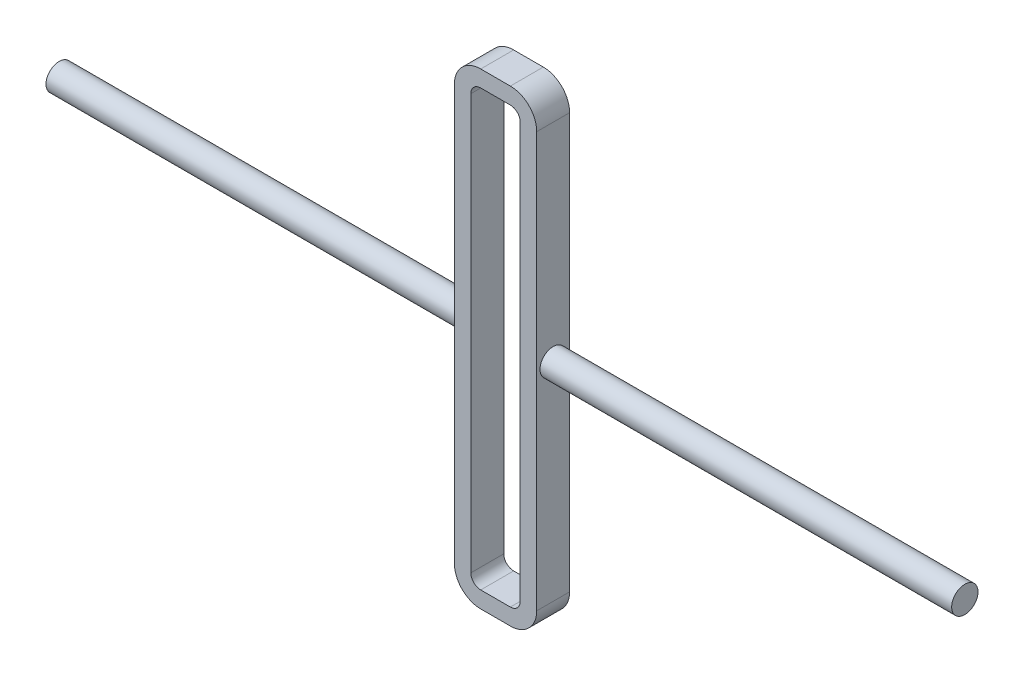
SolidWorks part; units mm, degrees
ref_plane "Front Plane" through (0, 0, 0) normal (0, 0, 1) x (1, 0, 0)
ref_plane "Top Plane" through (0, 0, 0) normal (0, 1, 0) x (1, 0, 0)
ref_plane "Right Plane" through (0, 0, 0) normal (1, 0, 0) x (0, 0, -1)
sketch "Sketch1" plane through (0, 0, 0) normal (0, 0, 1) x (1, 0, 0)
  line L0 (-4.5, 71) -> (4.5, 71)
  line L1 (-4.5, 66) -> (4.5, 66)
  line L2 (-7.5, 63) -> (-7.5, -63)
  line L3 (-4.5, -66) -> (4.5, -66)
  line L4 (7.5, 63) -> (7.5, -63)
  line L5 (-7.5, 66) -> (7.5, -66) construction
  line L6 (-7.5, -66) -> (7.5, 66) construction
  line L7 (12.5, 63) -> (12.5, -63)
  line L8 (-4.5, -71) -> (4.5, -71)
  line L9 (-12.5, 63) -> (-12.5, -63)
  arc A0 (-7.5, -63) -> (-4.5, -66) centre (-4.5, -63) ccw
  arc A1 (4.5, -66) -> (7.5, -63) centre (4.5, -63) ccw
  arc A2 (4.5, 66) -> (7.5, 63) centre (4.5, 63) cw
  arc A3 (-4.5, 66) -> (-7.5, 63) centre (-4.5, 63) ccw
  arc A4 (4.5, 71) -> (12.5, 63) centre (4.5, 63) cw
  arc A5 (4.5, -71) -> (12.5, -63) centre (4.5, -63) ccw
  arc A6 (-12.5, -63) -> (-4.5, -71) centre (-4.5, -63) ccw
  arc A7 (-4.5, 71) -> (-12.5, 63) centre (-4.5, 63) ccw
  point P0 (0, 0)
  dimension "D3" = 3
  dimension "D1" = 15
  dimension "D2" = 132
  dimension "D4" = 5
extrude "Boss-Extrude1" add sketch "Sketch1" along normal blind 10
sketch "Sketch2" plane through (12.5, 0, 0) normal (1, 0, 0) x (0, 0, -1)
  line L0 (0, -63) -> (0, 63) construction
  circle A0 centre (-5, 0) radius 4
  dimension "D1" = 8
  dimension "D2" = 5
extrude "Boss-Extrude2" add sketch "Sketch2" along normal blind 125
sketch "Sketch3" plane through (-12.5, 0, 0) normal (-1, 0, 0) x (0, 0, 1)
  line L0 (10, 63) -> (10, -63) construction
  circle A0 centre (5, 0) radius 4
  dimension "D1" = 8
  dimension "D2" = 5
extrude "Boss-Extrude3" add sketch "Sketch3" along normal blind 125
